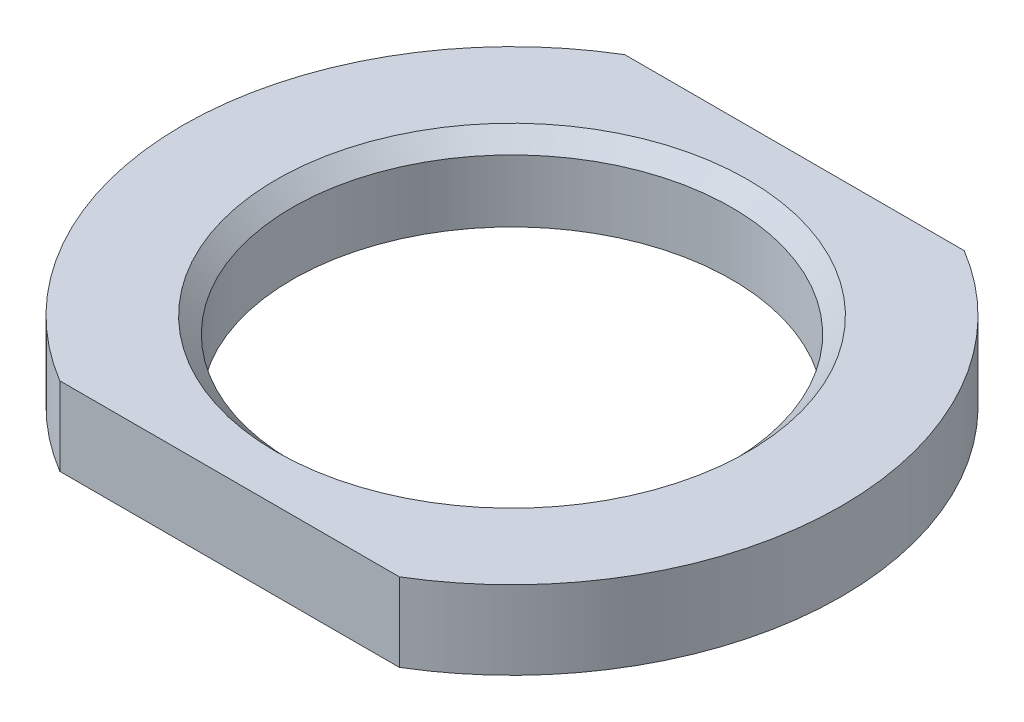
from build123d import *

# Parameters (mm, degrees)
BOSS_EXTRUDE1_DEPTH              = 5
M30X2_0_TAPPED_HOLE1_D           = 28
M30X2_0_TAPPED_HOLE1_DEPTH       = 70
M30X2_0_TAPPED_HOLE1_CSINK_D     = 30.05
M30X2_0_TAPPED_HOLE1_CSINK_ANGLE = 90
M30X2_0_TAPPED_HOLE1_TIP         = 8.412048666


with BuildPart() as part:
    # Sketch1 → Boss-Extrude1 (new body)
    with BuildSketch(Plane(origin=(0, 0, 0), x_dir=(1, 0, 0), z_dir=(0, 1, 0))):
        with BuildLine():
            Line((10.816653826, 18), (-10.816653826, 18))
            ThreePointArc((-10.816653826, 18), (-21, 0), (-10.816653826, -18))
            Line((-10.816653826, -18), (10.816653826, -18))
            ThreePointArc((10.816653826, -18), (18.277714988, -10.340461055), (21, 0))
            ThreePointArc((21, 0), (18.277714988, 10.340461055), (10.816653826, 18))
        make_face()
    extrude(amount=BOSS_EXTRUDE1_DEPTH)

    # M30x2.0 Tapped Hole1
    with Locations(Plane(origin=(0, 5, 0), x_dir=(1, 0, 0), z_dir=(0, 1, 0))):
        with Locations((0, 0)):
            CounterSinkHole(M30X2_0_TAPPED_HOLE1_D / 2, M30X2_0_TAPPED_HOLE1_CSINK_D / 2, depth=M30X2_0_TAPPED_HOLE1_DEPTH, counter_sink_angle=M30X2_0_TAPPED_HOLE1_CSINK_ANGLE)
            with Locations((0, 0, -(M30X2_0_TAPPED_HOLE1_DEPTH + M30X2_0_TAPPED_HOLE1_TIP / 2))):  # 118° drill point
                Cone(0, M30X2_0_TAPPED_HOLE1_D / 2, M30X2_0_TAPPED_HOLE1_TIP, mode=Mode.SUBTRACT)


solid = part.part
